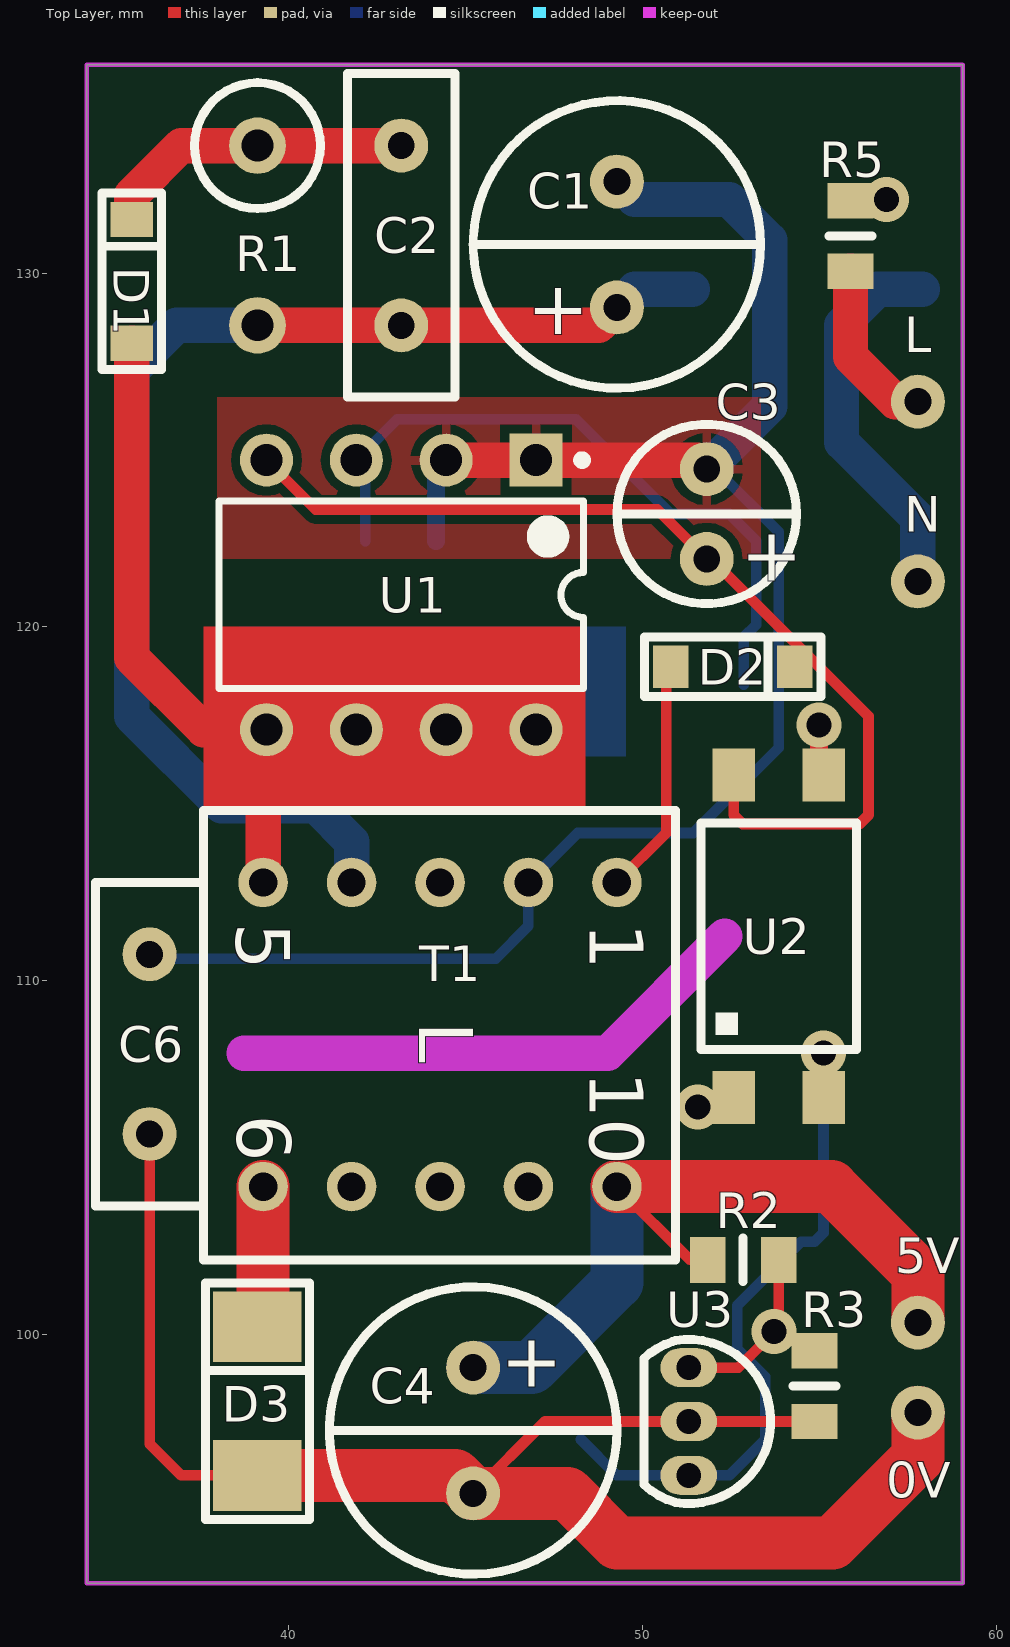
[diagram p0: Top Layer view]
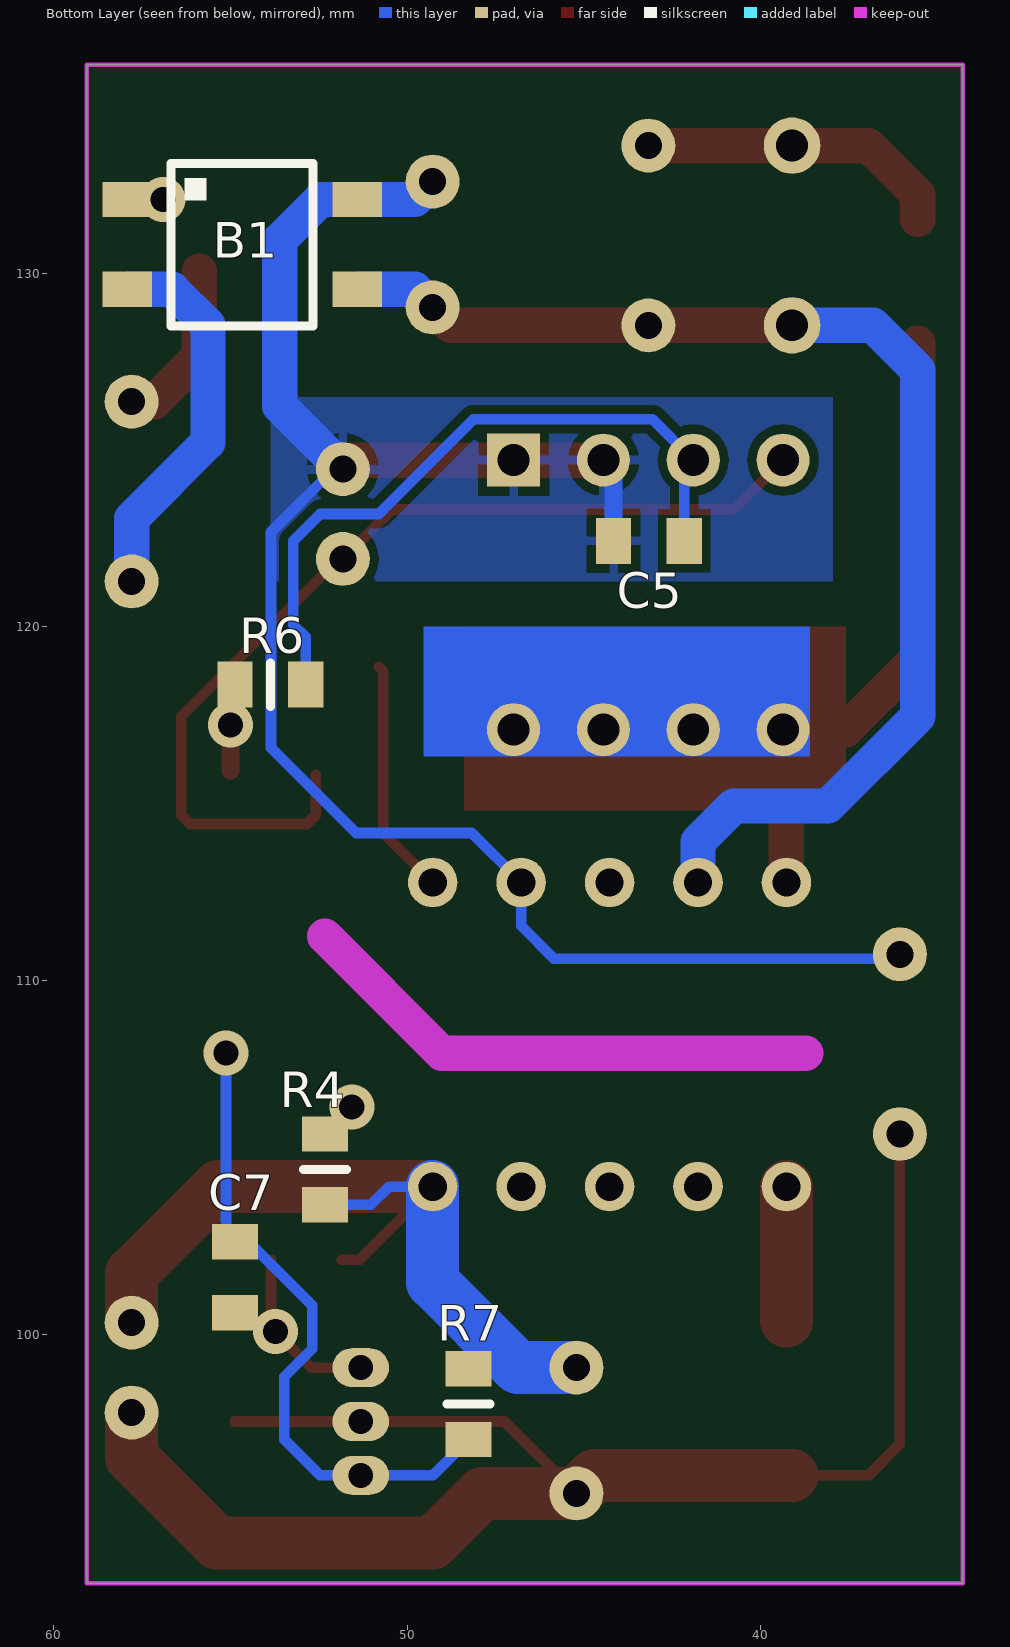
[diagram p1: Bottom Layer view, seen from below]
# Altium PCB MISC95264.PcbDoc
Units mm, origin at the board's own origin, x right, y up, seen from the top; angles counter-clockwise.
Board outline 24.77 x 42.93 mm, 2 copper layers (Top Layer, Bottom Layer); 22 components, 17 nets, 67 pads, 5 vias.

## Layer stack, top to bottom (the 12.6 mil dielectric is the usual default, probably not edited)
Top Layer: signal copper 0.0356
Dielectric: dielectric 0.32, FR-4, Dk 4.8
Bottom Layer: signal copper 0.0356

## Board outline
34.29,135.89 59.055,135.89 59.055,92.964 34.29,92.964

## Design rules (kind name [scope] priority, off if disabled: settings)
Clearance [All] p1: gap=0.254
PolygonConnect [All] p1: connectstyle=Relief reliefconductorwidth=0.254 reliefentries=4 polygonreliefangle="90 Angle"
RoutingVias [All] p1: holewidth=0.711 width=1.27 viastyle="Through Hole" minholewidth=0.711 minwidth=1.27 maxholewidth=0.711 maxwidth=1.27
SilkscreenOverComponentPads [All] p1: minsilkscreentomaskgap=0.254
SolderMaskExpansion [All] p1: expansion=0.102
Width [All] p1: maxlimit=1.5 minlimit=0.3 preferedwidth=1 minimp=50.000000 maximp=50.000000 favimp=50.000000
27 further rules are at their usual default settings.

## Components (designator, comment, footprint, x,y, rotation, side; value= is the part's Value field where it differs from the comment)
B1 "MB6S" SOP4 57.912,132.08 r180 bottom
C1 "4.7uF/400V" cap-8*14mm 49.276,129.032 r90 top
C2 "2.2nF/1KV" CAP_5mm 43.18,133.604 r270 top
C3 "10uF/25V" cap-5*12mm 51.816,121.92 r90 top
C4 "1000uF/10V" cap-8*14mm 45.212,99.06 r270 top
C5 "10nF" 0805_Cap 42.164,122.428 r0 bottom
C6 "1nF/1KV" CAP_5mm 36.068,105.664 r90 top
C7 "10nF" 0805_Cap 54.864,102.616 r270 bottom
D1 "F7" SOD-123 35.56,128.016 r90 top
D2 "F7" SOD-123 50.8,118.872 r0 top
D3 "SS34" DO_214AC/SMA 39.116,96.012 r90 top
R1 "33K/1W" 1W_Res_L 39.116,133.604 r270 top
R2 "1K" 0805_Res 53.848,102.108 r180 top
R3 "1K" 0805_Res 54.864,97.536 r90 top
R4 "470R" 0805_Res 52.324,105.664 r270 bottom
R5 "0R" 0805_Res 55.88,130.048 r90 top
R6 "8.2K" 0805_Res 52.864,118.364 r0 bottom
R7 "1K" 0805_Res 48.26,97.028 r90 bottom
T1 "EE13" EE13_5+5_L 49.276,112.776 r270 top
U1 "AP8012" DIP-8 43.18,120.904 r270 top
U2 "PC817" SOP4-PC817 53.848,111.252 r90 top
U3 "TL431" TO-92 51.308,99.06 r270 top

## Footprints (in the part's own frame and the unit in brackets; to place one, negate y for a bottom-side part, rotate by r counter-clockwise, add the part's x,y. Pads: shape width x height; smd on the part's side, far side on the other; paste and mask are expansions set on the pad)
1W_Res_L [mm]
  round 1.6 hole 0.9: 1(5.08,0) 2(0,0)
  silkscreen extent -1.78,-1.78 1.78,1.78
0805_Cap [mm]
  rect 1x1.3 smd: 1(0,0) 2(2,0)
0805_Res [mm]
  rect 1x1.3 smd: 1(0,0) 2(2,0)
  silkscreen extent 1,-0.61 1,0.61
cap-5*12mm [mil] "47uF/25V,diameter_5mm,height_12mm"
  round 60 hole 30: 1(0,0) 2(100,0)
  silkscreen extent -50,-100 150,100
cap-8*14mm [mil] "470uF/16V,diameter_8mm,height_14mm"
  round 60 hole 30: 1(0,0) 2(140,0)
  silkscreen extent -90,-160 230,160
CAP_5mm [mil] "10nF/1KV,Pin Distance 5mm"
  round 60 hole 30: 1(0,0) 2(200,0)
  silkscreen extent -80,-60 280,60
DIP-8 [mm] "DIP; 8 Leads; Row Spacing 7.62 mm; Pitch 2.54 mm"
  rect 1.5x1.5 hole 0.9: 1(-3.81,3.81)
  round 1.5 hole 0.9: 2(-3.81,1.27) 3(-3.81,-1.27) 4(-3.81,-3.81) 5(3.81,-3.81) 6(3.81,-1.27) 7(3.81,1.27) 8(3.81,3.81)
  silkscreen extent -3.93,-5.15 2.65,5.24, body extent -3.6,-5.15 3.6,5.15, height 5.08
DO_214AC/SMA [mm]
  rect 2x2.5 smd: 1(0,0) 2(4.2,0)
  silkscreen extent -1.24,-1.47 5.44,1.47
EE13_5+5_L [mm]
  round 1.4 hole 0.8: 1(0,0) 2(0,-2.5) 3(0,-5) 4(0,-7.5) 5(0,-10) 6(8.6,-10) 7(8.6,-7.5) 8(8.6,-5) 9(8.6,-2.5) 10(8.6,0)
  silkscreen extent -2.03,-11.68 10.67,1.65
SOD-123 [mm]
  rect 1x1.2 smd: 1(0,0) 2(3.5,0)
  silkscreen extent -0.74,-0.84 4.24,0.84
SOP4 [mm]
  rect 1.4x1 smd: 1(0,0) 2(0,-2.54) 3(6.5,-2.54) 4(6.5,0)
  silkscreen extent 1.24,-3.58 5.26,1.02
SOP4-PC817 [mm] "SOP4 for PC817"
  rect 1.5x1.2 smd: 1(-4.56,1.27) 2(-4.56,-1.27) 3(4.56,-1.27) 4(4.56,1.27)
  silkscreen extent -3.2,-2.2 3.2,2.2
TO-92 [mm] "TL431,S8550,S8050"
  oval 1.1x1.6 hole 0.7: 1(0,0) 2(1.524,0) 3(3.048,0)
  silkscreen extent -0.79,-1.27 3.84,2.31

## Part data
B1: "600V 0.8A Bridge Rectifiers"
C1 C3 C4: library part "Cap Pol"
C2 C5 C6 C7: library part Cap
D1 D2 D3: library part Diode
R1 R2 R3 R4 R5 R6 R7: library part Res
T1: library part "Flyback transformer-1"
U1: "5W Flyback SMPS Controller"
U2: "Device Specification For PhotoCoupler"
U3: "Adjustable Precision Shunt Regulator"

## Free pads (board coordinates)
  round 1.524 hole 0.762: 0(57.785,100.33) 1(57.785,97.79) 2(57.785,126.365) 3(57.785,121.285)

## Via types
v1: diameter 1.27, hole 0.711, Top Layer to Bottom Layer, tented both sides, 5 vias

## Nets (pads, with @x,y where several pads share a name; then routed paths per layer and width w, separated by ;. In a path a pad name is that pad's centre, name@x,y a point inside that pad or via, vN(x,y) a via of type N, cw(c..) or ccw(c..) an arc to the next point about the centre after c; other vN are vias at no path point)
5V: C4.1 pad.0 R2.2 R4.2 R7.2 T1.10 | length 25.4
  Top Layer w0.3: T1.10 51.344,102.108 R2.2
  Top Layer w1.5: T1.10 55.336,104.176 57.785,101.727 pad.0
  Bottom Layer w0.3: T1.10 50.51,104.176 51.022,103.664 R4.2
  Bottom Layer w1.5: C4.1 46.863,99.06 49.276,101.473 T1.10
GND: C4.2 C6.1 D3.1 pad.1 R3.1 U3.2 | length 44.4
  Top Layer w0.3: C6.1 36.068,96.901 36.957,96.012 D3.1 ; C4.2 47.244,97.536 U3.2 R3.1
  Top Layer w1.5: D3.1 44.704,96.012 C4.2 47.879,95.504 49.276,94.107 55.372,94.107 57.785,96.52 pad.1
HGND: B1.4 C1.2 C3.2 C5.2 C6.2 T1.2 U1.1 U1.2 | length 52.2
  Top Layer w1: U1.2 51.562,124.714 C3.2
  Bottom Layer w0.3: C6.2@35.56,110.744 C6.2 36.195,110.617 45.847,110.617 46.776,111.546 T1.2 48.173,114.173 51.435,114.173 53.848,116.586 53.848,122.682 C3.2@52.07,124.46
  Bottom Layer w0.5: C5.2 44.164,124.428 U1.2
  Bottom Layer w1: C1.2 49.784,132.08 B1.4 52.451,132.08 53.594,130.937 53.594,126.238 C3.2
L: pad.2 R5.1 | length 4.8
  Top Layer w1: R5.1 55.88,127.635 57.15,126.365 pad.2
N: B1.2 pad.3 | length 10.8
  Bottom Layer w1: pad.3 57.785,123.063 55.626,125.222 55.626,128.524 56.642,129.54 B1.2
NetB1_1: B1.1 R5.2
  other v1: 56.896,132.08
NetB1_3: B1.3 C1.1 C2.2 R1.1 T1.4 | length 35.4
  Top Layer w1: R1.1 C2.2 48.768,128.524 C1.1
  Bottom Layer w1: R1.1 36.83,128.524 35.56,127.254 35.56,117.475 38.1,114.935 40.767,114.935 41.776,113.926 T1.4 ; C1.1 49.784,129.54 B1.3
NetC2_1: C2.1 D1.2 R1.2 | length 8.9
  Top Layer w1: D1.2 35.56,132.207 36.957,133.604 R1.2 C2.1
NetC3_1: C3.1 D2.2 U1.4 U2.4 | length 28
  Top Layer w0.3: U1.4 40.767,123.317 50.419,123.317 C3.1 ; C3.1@51.752,121.856 52.006,121.856 56.388,117.475 56.388,114.681 56.134,114.427 52.832,114.427 52.578,114.681 U2.4
NetC5_1: C5.1 R6.1 U1.3 | length 19.8
  Bottom Layer w0.3: C5.1 42.164,124.46 U1.3 43.064,125.868 48.122,125.868 50.8,123.19 52.451,123.19 53.213,122.428 53.213,120.061 52.864,119.712 R6.1
NetC7_1: C7.1 R7.1 U2.2 U3.3 | length 18.5
  Bottom Layer w0.3: R7.1 49.276,96.012 U3.3 52.451,96.012 53.467,97.028 53.467,98.806 52.682,99.591 52.682,100.815 54.483,102.616 C7.1 55.118,102.87 v1(55.118,107.95)
NetC7_2: C7.2 R2.1 R3.2 U3.1 | length 4.9
  Top Layer w0.3: U3.1 52.705,99.06 v1(53.721,100.076) 53.848,100.203 R2.1
NetD1_1: D1.1 T1.5 U1.5 U1.6 U1.7 U1.8 | length 25.5
  Top Layer w1: D1.1 35.56,119.126 37.592,117.094 U1.5 ; T1.5 39.276,117 U1.5 ; U1.8 U1.7 U1.6 U1.5
NetD2_1: D2.1 T1.1 | length 6.7
  Top Layer w0.3: T1.1 50.673,114.173 50.673,118.745 D2.1
NetD3_2: D3.2 T1.6 | length 3.8
  Top Layer w1.5: D3.2@39.276,100.372 T1.6
NetR4_1: R4.1 U2.1
  other v1: 51.562,106.426
NetR6_2: R6.2 U2.3 | length 1.3
  Top Layer w0.5: U2.3@54.991,115.939 v1(54.991,117.221)
pads on no net: T1.3 T1.7 T1.8 T1.9

## Polygon pours and split planes (outlines as drawn)
HGND on Bottom Layer "Bottom Layer-No Net" (solid, pour order 1000): 37.973,126.492 37.973,121.285 53.848,121.285 53.848,126.492
HGND on Top Layer "Bottom Layer-No Net" (solid, pour order 1001): 37.973,126.492 37.973,121.92 53.34,121.92 53.34,126.492

## Keep-outs
Keep-Out Layer:
  lines w0.127: 34.29,92.964 59.055,92.964 59.055,135.89 34.29,135.89 34.29,92.964
  lines w1: 38.735,107.95 49.022,107.95 52.324,111.252

## Other copper
Top Layer:
  rectangle net NetD1_1: 37.592,114.808 48.387,120.015
Bottom Layer:
  rectangle net NetD1_1: 38.608,116.332 49.53,120.015

## Silkscreen, mask and mechanical layers (free items; w line width, h text height)
Top Overlay:
  text "L" at 57.404,127.762 h1.02
  text "N" at 57.404,122.682 h1.02
  text "5V" at 57.15,101.727 h1.02
  text "0V" at 56.896,95.377 h1.02